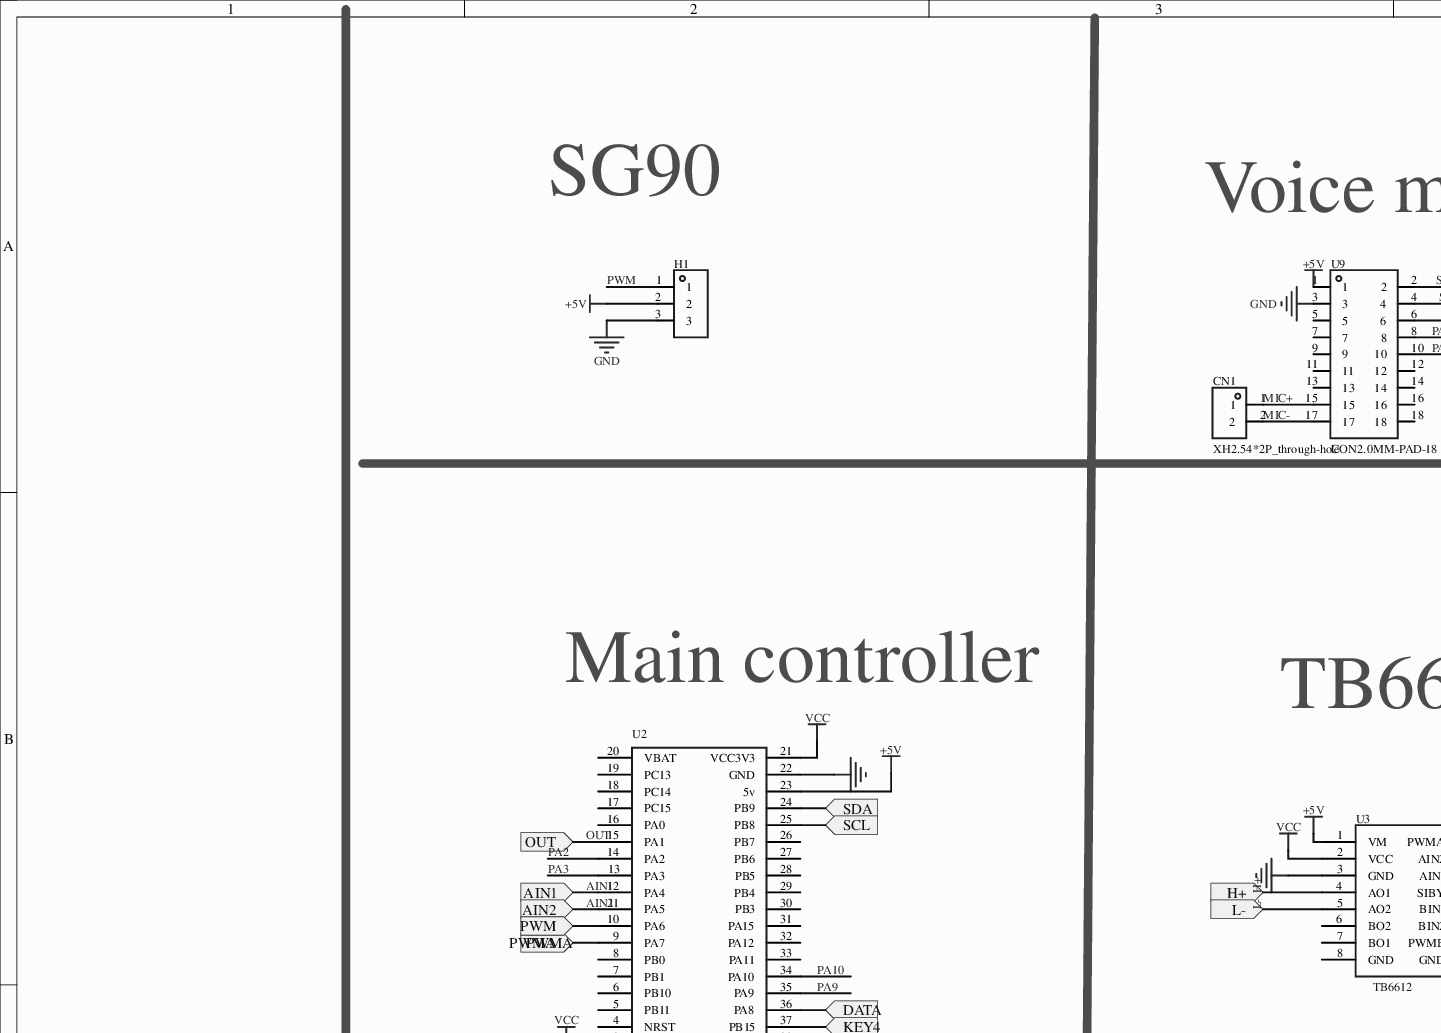
[diagram p0: MISC51940-3.schdoc, top left]
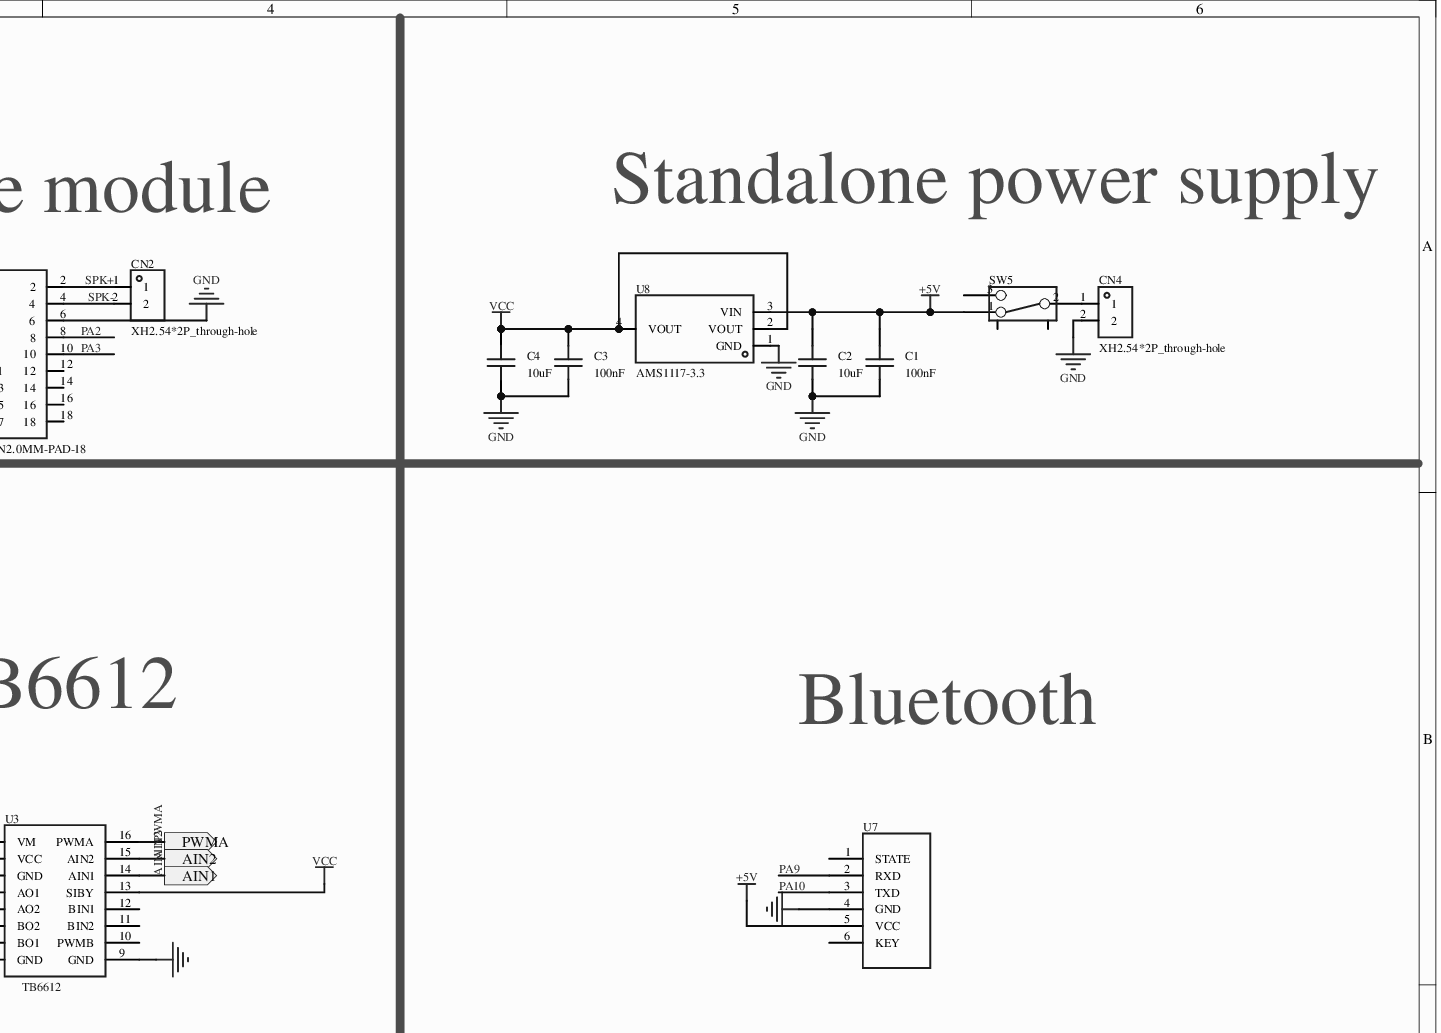
[diagram p1: MISC51940-3.schdoc, top right]
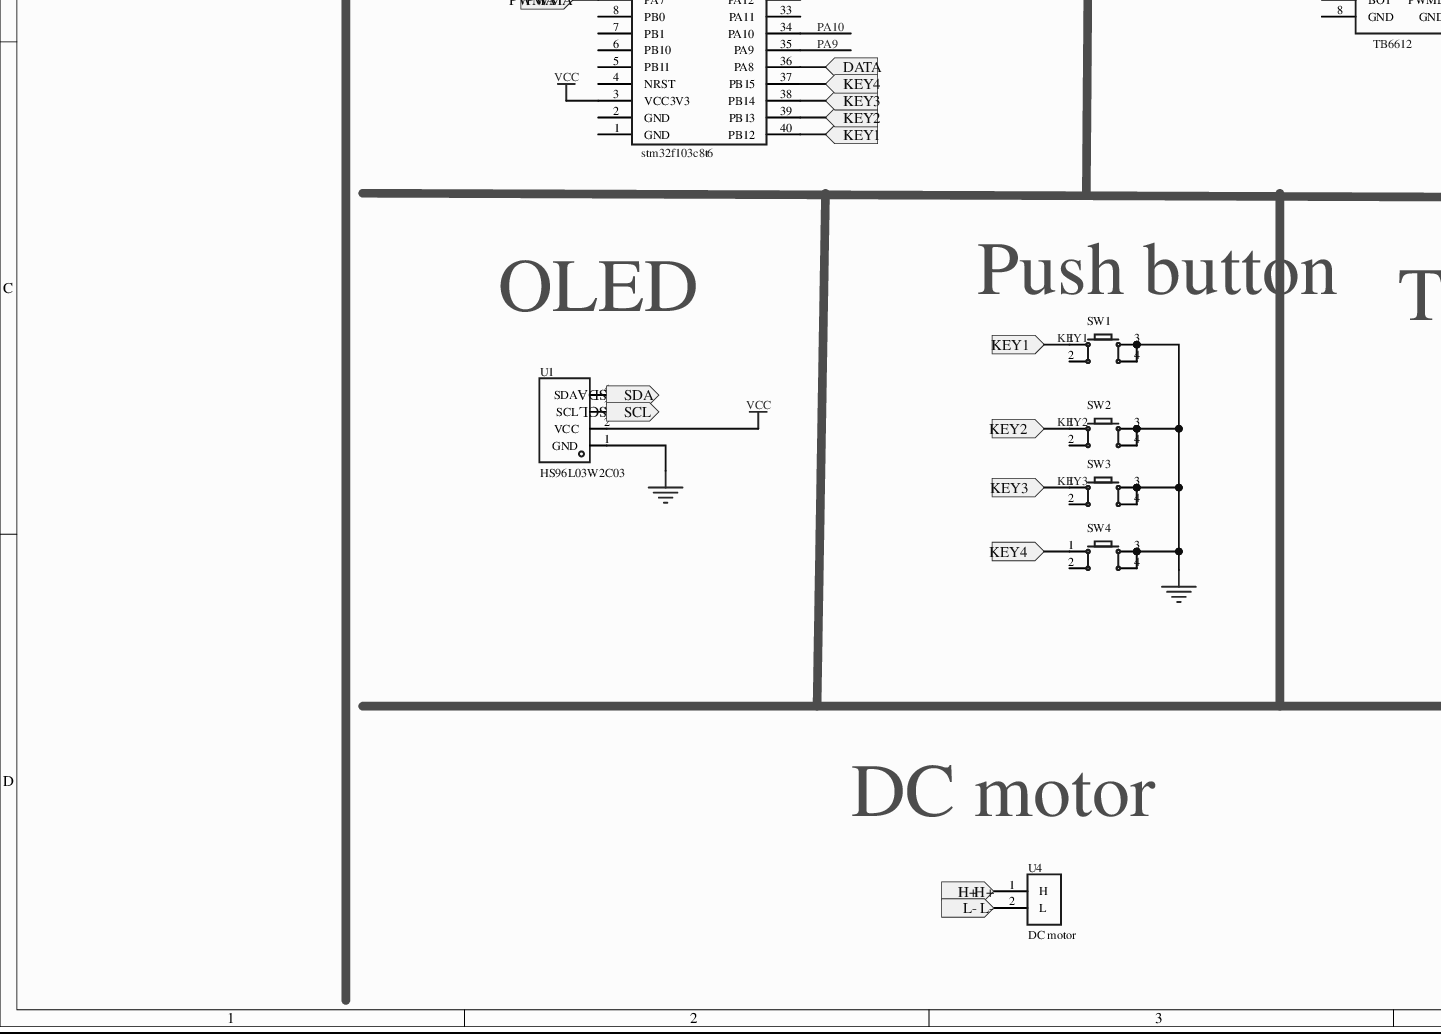
[diagram p2: MISC51940-3.schdoc, bottom left]
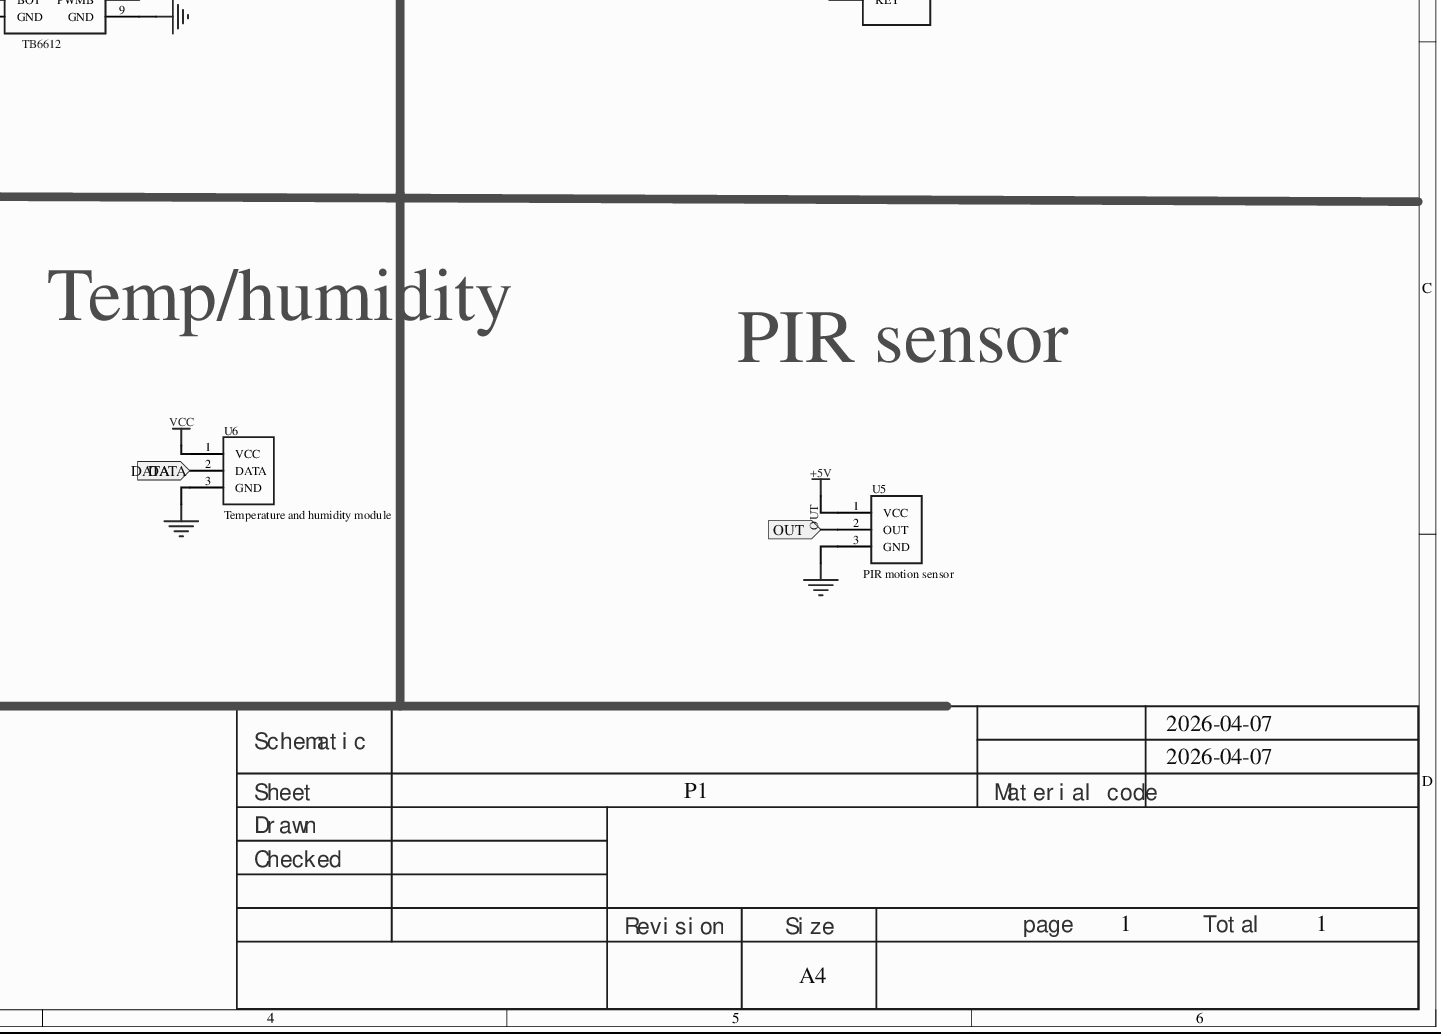
[diagram p3: MISC51940-3.schdoc, bottom right]
# Altium project MISC51940-2.PrjPcb
1 sheet, 22 parts. Net scope: flat (ports and power ports of the same name join across sheets).
Board file: MISC51940.pcbdoc

## Sheet MISC51940-3.schdoc
size 420 x 297 mm; Version: V1.0; @Project Name: MISC51940; @Page Count: 1; @Update Date: 2026-04-07; @Create Date: 2026-04-07; @Schematic Name: MISC51940; @Page No: 1

### Parts
C1  100nF  [C0603]
C2  10uF  [C0603]
C3  100nF  [C0603]
C4  10uF  [C0603]
CN1  XH2.54*2P_through-hole  [CONN-TH_2P-P2.50-XH2.54-2P]
CN2  XH2.54*2P_through-hole  [CONN-TH_2P-P2.50-XH2.54-2P]
CN4  XH2.54*2P_through-hole  [CONN-TH_2P-P2.50-XH2.54-2P]
H1  (no value)  [HDR-TH_3P-P2.54-V-F]
SW1  (no value)  [按键]
SW2  (no value)  [按键]
SW3  (no value)  [按键]
SW4  (no value)  [按键]
SW5  (no value)  [拨动开关]
U1  HS96L03W2C03  [OLED-TH_L27.8-W27.2-P2.54_C9900033791]
U2  (no value)  [STM32]
U3  (no value)  [电机驱动模块]
U4  Device: DC motor  [直流电机]
U5  Device: PIR motion sensor  [人体红外模块]
U6  Device: Temperature and humidity module  [DHT11温湿度]
U7  (no value)  [蓝牙HC-08]
U8  AMS1117-3.3  [SOT-223-3_L6.5-W3.4-P2.30-LS7.0-BR]
U9  CON2.0MM-PAD-18  [CONN-TH_18P-P2.00_C9900078766]

### Ports
AIN1 (in), AIN1 (out), AIN2 (in), AIN2 (out), DATA (in), H+ (in), KEY1 (in), KEY2 (in), KEY3 (in), KEY4 (in), L- (in), OUT (in), PWM (in), PWMA (in), PWMA (out), SCL (in), SCL (out), SDA (in), SDA (out)

### Nets
+5V: C1.2 C2.2 H1.2 SW5.1 U2.23(5v) U3.1(VM) U5.1(VCC) U7.5(VCC) U8.3(VIN) U9.1
GND: C1.1 C2.1 C3.1 C4.1 CN4.2 H1.3 SW1.3 SW1.4 SW2.3 SW2.4 SW3.3 SW3.4 SW4.3 SW4.4 U1.1(GND) U2.22(GND) U3.3(GND) U3.9(GND) U5.3(GND) U6.3(GND) U7.4(GND) U8.1(GND) U9.3 U9.6
VCC: C3.2 C4.2 U1.2(VCC) U2.3(VCC3V3) U2.21(VCC3V3) U3.2(VCC) U3.13(SIBY) U6.1(VCC) U8.2(VOUT) U8.4(VOUT)
AIN1: U2.12(PA4) U3.14(AIN1) ; port AIN1
AIN2: U2.11(PA5) U3.15(AIN2) ; port AIN2
DATA: U2.36(PA8) U6.2(DATA) ; port DATA
H+: U3.4(AO1) U4.1(H) ; port H+
KEY1: SW1.1 U2.40(PB12) ; port KEY1
KEY2: SW2.1 U2.39(PB13) ; port KEY2
KEY3: SW3.1 U2.38(PB14) ; port KEY3
L-: U3.5(AO2) U4.2(L) ; port L-
MIC+: CN1.1 U9.15
MIC-: CN1.2 U9.17
OUT: U2.15(PA1) U5.2(OUT) ; port OUT
PA2: U2.14(PA2) U9.8
PA3: U2.13(PA3) U9.10
PA9: U2.35(PA9) U7.2(RXD)
PA10: U2.34(PA10) U7.3(TXD)
PWM: H1.1
PWMA: U2.9(PA7) U3.16(PWMA) ; port PWMA
SCL: U1.3(SCL) U2.25(PB8) ; port SCL
SDA: U1.4(SDA) U2.24(PB9) ; port SDA
SPK+: CN2.1 U9.2
SPK-: CN2.2 U9.4
NetCN4_1: CN4.1 SW5.2
NetSW4_1: SW4.1 U2.37(PB15) ; port KEY4
NetU2_10: U2.10(PA6) ; port PWM

Not connected (* = marked no-connect by the designer): SW1 2; SW2 2; SW3 2; SW4 2; SW5 3 4 5; U2 1(GND) 2(GND) 4(NRST) 5(PB11) 6(PB10) 7(PB1) 8(PB0) 16(PA0) 17(PC15) 18(PC14) 19(PC13) 20(VBAT) 26(PB7) 27(PB6) 28(PB5) 29(PB4) 30(PB3) 31(PA15) 32(PA12) 33(PA11); U3 6(BO2) 7(BO1) 8(GND) 10(PWMB) 11(BIN2) 12(BIN1); U7 1(STATE) 6(KEY); U9 5 7 9 11 12 13 14 16 18

### Notes on the sheet
- SG90
- Voice module
- Standalone power supply
- (near U2) Main controller
- TB6612
- Bluetooth
- (near SW1) Push button
- OLED
- Temp/humidity
- PIR sensor
- (near U4) DC motor
- 2026-04-07
- Schematic
- Sheet
- P1
- Material code
- Checked
- Drawn
- Revision
- Size
- A4
- page
- 1
- Total

### Library data of the parts
C1-C4 = CAP_0603: Symbol: Capacitance; ConvertToPcb: yes; ModelId: ac125912035d415993ca9572d50418b10819f05c4eef4c71ace90d822a990e87; ModelName: C0603_L1.6-W0.8-H0.8; ModelTransform: 62.992,31.496,0,0,0,0,0,0,0; Device: CAP_0603; AddInBom: yes; Supplier Footprint: 0603; FootprintName: C0603
  C1 C3: Value: 100nF
  C2 C4: Value: 10uF
CN1 CN2 CN4 = XH2.54*2P_直插: 3D Model: 325c595e30db4df8abe76612dd40b0fa0819f05c4eef4c71ace90d822a990e87; 3D Model Transform: 295.275,228.346,0,180,0,0,-0.002,-20.079,-137.795; AddInBom: yes; Symbol: XH2.54*2P_through-hole; Device: XH2.54*2P_through-hole; LCSC Part Name: XH2.54*2P_直插; Supplier Part: C9900008615; Manufacturer Part: XH2.54*2P_直插; Supplier Footprint: XH2.54_2P; JLCPCB Part Class: Extended Part; Supplier: LCSC; ConvertToPcb: yes; FootprintName: CONN-TH_2P-P2.50-XH2.54-2P; ModelName: CONN-TH_2P-P2.50-XH2.54-2P
H1 = HDR-F_2.54_1x3P: Symbol: PM254V-11-03-H85; ConvertToPcb: yes; ModelId: f3b3cc5aae9641bf9e56fc160cef875b0819f05c4eef4c71ace90d822a990e87; ModelName: HDR2.54-F-LI-1X3P; ModelTransform: 299.9994,100,0,0,0,0,0,0,-118.11; Device: HDR-F_2.54_1x3P; AddInBom: yes; SupplierPart: C541850; Supplier Footprint: 插件; FootprintName: HDR-TH_3P-P2.54-V-F
SW1-SW4 = Key_SMD_6x6x6.5: Symbol: Tactile push button; ConvertToPcb: yes; ModelId: fbf4ceca6c4742d48614ab6a891ef981; ModelName: SW-SMD_4P-L6.0-W6.0-P4.50-LS11.0; ModelTransform: 330.708,251.968,0,0,0,0,0,-0.005,0; Device: Key_SMD_6x6x6.5; AddInBom: yes; Supplier Footprint: SMD; FootprintName: Push button
SW5 = 拨动开关_正: Symbol: Toggle switch; Device: Toggle switch_positive; 3D Model: 4321fe59a4074cbfb4989553f297c68f0819f05c4eef4c71ace90d822a990e87; 3D Model Transform: 370.09,208.7,472.35,0,0,0,0,0,-110; ConvertToPcb: yes; ModelName: SW-TH_SS-12D02-VG4; Supplier Footprint: 插件; AddInBom: yes; FootprintName: Toggle switch
U1 = HS96L03W2C03: Main controller: SSD1315; interface: I2C; size (inch): 0.96; resolution: 128x64;; Manufacturer: HS(汉昇); AddInBom: yes; ModelId: c6b423183c2f4cf5a163f75f8ad52fae; ModelTransform: 1070.864,1094.486,0,0,0,0,0,-468.503,0; Symbol: HS96L03W2C03; Device: HS96L03W2C03; LCSC Part Name: 0.96寸OLED显示屏窄白光IIC; SupplierPart: C5248080; ManufacturerPart: HS96L03W2C03; Supplier Footprint: -; JLCPCB Part Class: Extended library; Datasheet: https://atta.szlcsc.com/upload/public/pdf/source/20230627/763D01F79A90007632F098068C7C8AD9.pdf; Supplier: LCSC; ConvertToPcb: yes; FootprintName: OLED-TH_L27.8-W27.2-P2.54_C9900033791; ModelName: OLED-TH_L27.8-W27.2-P2.54_C9900033791; Main Control Chip: SSD1315; Interface Type: I2C; Size: 0.96; Pixel Resolution: 128x64; Operating Temperature: -40℃~+70℃
U2 = stm32f103c8t6: AddInBom: yes; Device: stm32f103c8t6; Symbol: stm32f103c8t6; ConvertToPcb: yes
U3 = TB6612: AddInBom: yes; Device: TB6612; Symbol: TB6612; ConvertToPcb: yes
U4 = 直流电机: AddInBom: yes; Symbol: DC motor; ConvertToPcb: yes
U5 = 人体红外传感器: AddInBom: yes; Symbol: PIR motion sensor; ConvertToPcb: yes
U6 = 温湿度模块: AddInBom: yes; Symbol: Temperature and humidity module; ConvertToPcb: yes
U7 = 蓝牙HC-08: Device: Bluetooth HC-08; AddInBom: yes; Symbol: Bluetooth HC-08; ConvertToPcb: yes; FootprintName: Bluetooth HC-08
U8 = AMS1117-3.3_C6186: Output type: fixed; operating voltage: 15V; output voltage: 3.3V; output current: 1A; PSRR: 72dB@(120Hz); output polarity: positive;; Manufacturer: AMS; AddInBom: yes; ModelId: 925194bf9823436183a3e0b978a8d0760819f05c4eef4c71ace90d822a990e87; ModelName: SOT-223-4P_L6.5-W3.5-H1.6-LS7.0-P2.30; ModelTransform: 279.89794,255.905,0,180,0,0,-3.9385,-0.0005,0; Voltage Dropout: 1.1V@(800mA); standby current: 5mA; Noise: 0.003%Vout; Number of Outputs: 1; Symbol: AMS1117-3.3; Device: AMS1117-3.3_C6186; LCSC Part Name: 3.3V 1A 15V; SupplierPart: C6186; ManufacturerPart: AMS1117-3.3; Supplier Footprint: SOT-223; JLCPCB Part Class: Basic Part; Datasheet: https://item.szlcsc.com/datasheet/AMS1117-3.3/6652.html; Supplier: LCSC; ConvertToPcb: yes; FootprintName: SOT-223-3_L6.5-W3.4-P2.30-LS7.0-BR; Output Type: Fixed; Voltage - Supply: 15V; Output Voltage: 3.3V; Output Current: 1A; Power Supply Rejection Ratio (PSRR): 72dB@(120Hz); Features: Overcurrent protection; thermal shutdown; Operating Temperature: -40℃~+125℃; Output Configuration: Positive
U9 = CON2.0MM-PAD-18: 3D Model: 07100c6dd3a4442ea12d6f5a4e41c4c80819f05c4eef4c71ace90d822a990e87; 3D Model Transform: 787.7937,374.015,0,0,0,0,0,-14.961,-118.11; AddInBom: yes; Symbol: CON2.0MM-PAD-18; Device: CON2.0MM-PAD-18; LCSC Part Name: CON2.0MM-PAD-18; Supplier Part: C9900078766; Manufacturer Part: CON2.0MM-PAD-18; Supplier Footprint: TH-2*9P-2.0; JLCPCB Part Class: Extended Part; Supplier: LCSC; ConvertToPcb: yes; FootprintName: CONN-TH_18P-P2.00_C9900078766; ModelName: CONN-TH_18P-P2.00_C9900078766